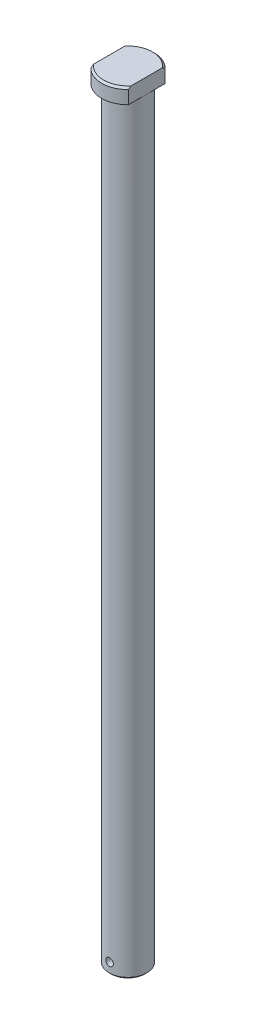
SolidWorks part; units mm, degrees
material "Plain Carbon Steel"
ref_plane "Front Plane" through (0, 0, 0) normal (0, 0, 1) x (1, 0, 0)
ref_plane "Top Plane" through (0, 0, 0) normal (0, 1, 0) x (1, 0, 0)
ref_plane "Right Plane" through (0, 0, 0) normal (1, 0, 0) x (0, 0, -1)
sketch "Sketch1" plane through (0, 0, 0) normal (0, 0, 1) x (1, 0, 0)
  line L0 (0, -318.9881) -> (0, 15630.419) construction
  line L1 (0, 0) -> (7, 0)
  line L2 (7, 0) -> (7, -4)
  line L3 (7, -4) -> (5, -4)
  line L4 (5, -4) -> (5, -207)
  line L5 (5, -207) -> (0, -207)
  line L6 (0, -207) -> (0, 0)
  dimension "D1" = 7
  dimension "D2" = 5
  dimension "D3" = 4
  dimension "D4" = 207
revolve "Revolve1" add sketch "Sketch1" angle 360 about L0
chamfer "Chamfer1" distance 0.5 angle 45 2 edges at (5, -207, 0) (7, 0, 0)
sketch "Sketch2" plane through (0, 0, 0) normal (0, 0, 1) x (1, 0, 0)
  line L0 (0, -1000) -> (0, 49000) construction
  line L1 (-5, -4) -> (5, -4) construction
  circle A0 centre (0, -204) radius 1
  dimension "D2" = 2
  dimension "D1" = 200
extrude "Cut-Extrude1" cut sketch "Sketch2" against normal through all both and the other way through all
sketch "Sketch3" plane through (0, 0, 0) normal (0, 0, 1) x (1, 0, 0)
  line L0 (6.5, 0) -> (-6.5, 0) construction
  line L1 (-7, -4) -> (-5, -4)
  line L2 (-7, -4) -> (-7, 0)
  line L3 (-7, 0) -> (-5, 0)
  line L4 (-5, -4) -> (-5, 0)
  dimension "D1" = 2
extrude "Cut-Extrude2" cut sketch "Sketch3" against normal through all both and the other way through all
sketch "Sketch4" plane through (0, 0, 0) normal (0, 0, 1) x (1, 0, 0)
  line L0 (6.5, 0) -> (-5, 0) construction
  line L1 (7, -4) -> (5, -4)
  line L2 (7, -4) -> (7, 0)
  line L3 (7, 0) -> (5, 0)
  line L4 (5, -4) -> (5, 0)
  dimension "D1" = 2
extrude "Cut-Extrude3" cut sketch "Sketch4" against normal through all both and the other way through all
